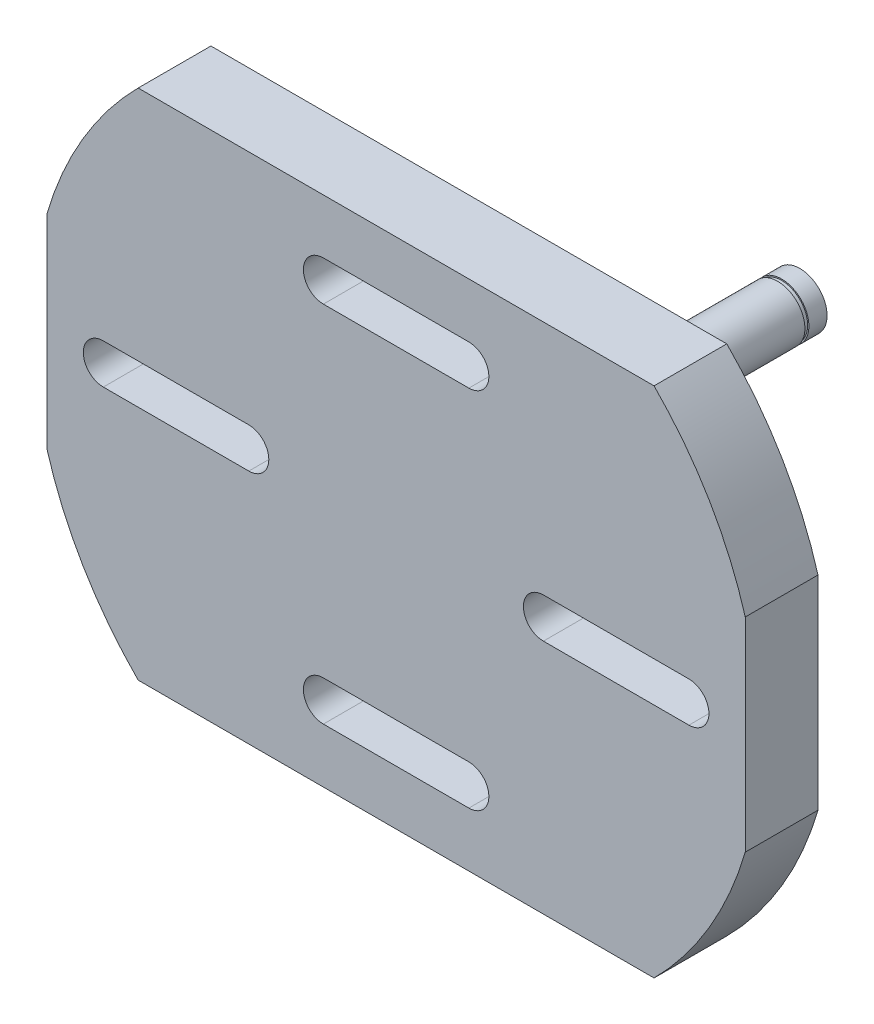
SolidWorks part; units mm, degrees
ref_plane "前视基准面" through (0, 0, 0) normal (0, 0, 1) x (1, 0, 0)
ref_plane "上视基准面" through (0, 0, 0) normal (0, 1, 0) x (1, 0, 0)
ref_plane "右视基准面" through (0, 0, 0) normal (1, 0, 0) x (0, 0, -1)
sketch "草图1" plane through (0, 0, 0) normal (0, 1, 0) x (1, 0, 0)
  line L0 (0, 0) -> (0, -30119.4069) construction
  line L1 (0, 111) -> (-7.5, 111)
  line L2 (-7.5, 111) -> (-7.5, 106)
  line L3 (-7.5, 106) -> (-7.15, 106)
  line L4 (-7.15, 106) -> (-7.15, 104.9)
  line L5 (-7.15, 104.9) -> (-7.5, 104.9)
  line L6 (-7.5, 104.9) -> (-7.5, 60)
  line L7 (-7.5, 60) -> (-10, 60)
  line L8 (-10, 60) -> (-10, 55)
  line L9 (-30, 20) -> (-100, 20)
  line L10 (-100, 20) -> (-100, 0)
  line L11 (-100, 0) -> (0, 0)
  line L12 (0, 111) -> (0, 0)
  line L13 (-10, 55) -> (-30, 55)
  line L14 (-30, 55) -> (-30, 20)
  dimension "D1" = 15
  dimension "D2" = 51
  dimension "D3" = 20
  dimension "D4" = 14.3
  dimension "D5" = 1.1
  dimension "D6" = 5
  dimension "D7" = 20
  dimension "D8" = 60
  dimension "D9" = 200
  dimension "D10" = 60
  dimension "D11" = 5
revolve "旋转1" add sketch "草图1" angle 360 about L0
sketch "草图3" plane through (0, 0, -20) normal (0, 0, -1) x (-1, 0, 0)
  line L0 (-20, 50) -> (20, 50) construction
  line L1 (-20, 55.5) -> (20, 55.5)
  line L2 (-20, 44.5) -> (20, 44.5)
  line L3 (-40.5, 0) -> (-80.5, 0) construction
  line L6 (-40.5, -5.5) -> (-80.5, -5.5)
  line L7 (-40.5, 5.5) -> (-80.5, 5.5)
  arc A0 (-20, 55.5) -> (-20, 44.5) centre (-20, 50) ccw
  arc A1 (20, 44.5) -> (20, 55.5) centre (20, 50) ccw
  circle A3 centre (0, 0) radius 30 construction
  arc A7 (-40.5, -5.5) -> (-40.5, 5.5) centre (-40.5, 0) ccw
  arc A8 (-80.5, 5.5) -> (-80.5, -5.5) centre (-80.5, 0) ccw
  point P2 (0, 50)
  point P12 (-60.5, 0)
  point P17 (-58.1158, 0)
  dimension "D1" = 20
  dimension "D2" = 5.5
  dimension "D4" = 40
  dimension "D5" = 5
  dimension "D6" = 5.5
  dimension "D3" = 40
extrude "切除-拉伸1" cut sketch "草图3" against normal through all
mirror "镜向1" about plane through (0, 0, 0) normal (1, 0, 0) of "切除-拉伸1"
mirror "镜向2" about plane through (0, 0, 0) normal (0, 1, 0) of "切除-拉伸1"
sketch "草图4" plane through (0, 0, -20) normal (0, 0, -1) x (-1, 0, 0)
  line L0 (20, 55.5) -> (-20, 55.5) construction
  line L1 (-96, -70.5) -> (96, -70.5)
  line L2 (-96, -70.5) -> (-96, 70.5)
  line L3 (-96, 70.5) -> (96, 70.5)
  line L4 (96, -70.5) -> (96, 70.5)
  line L5 (-96, -70.5) -> (96, 70.5) construction
  line L6 (-96, 70.5) -> (96, -70.5) construction
  arc A0 (-80.5, 5.5) -> (-80.5, -5.5) centre (-80.5, 0) ccw construction
  point P0 (0, 0)
  dimension "D2" = 10
  dimension "D1" = 15
extrude "切除-拉伸2" cut sketch "草图4" against normal through all flip side to cut
